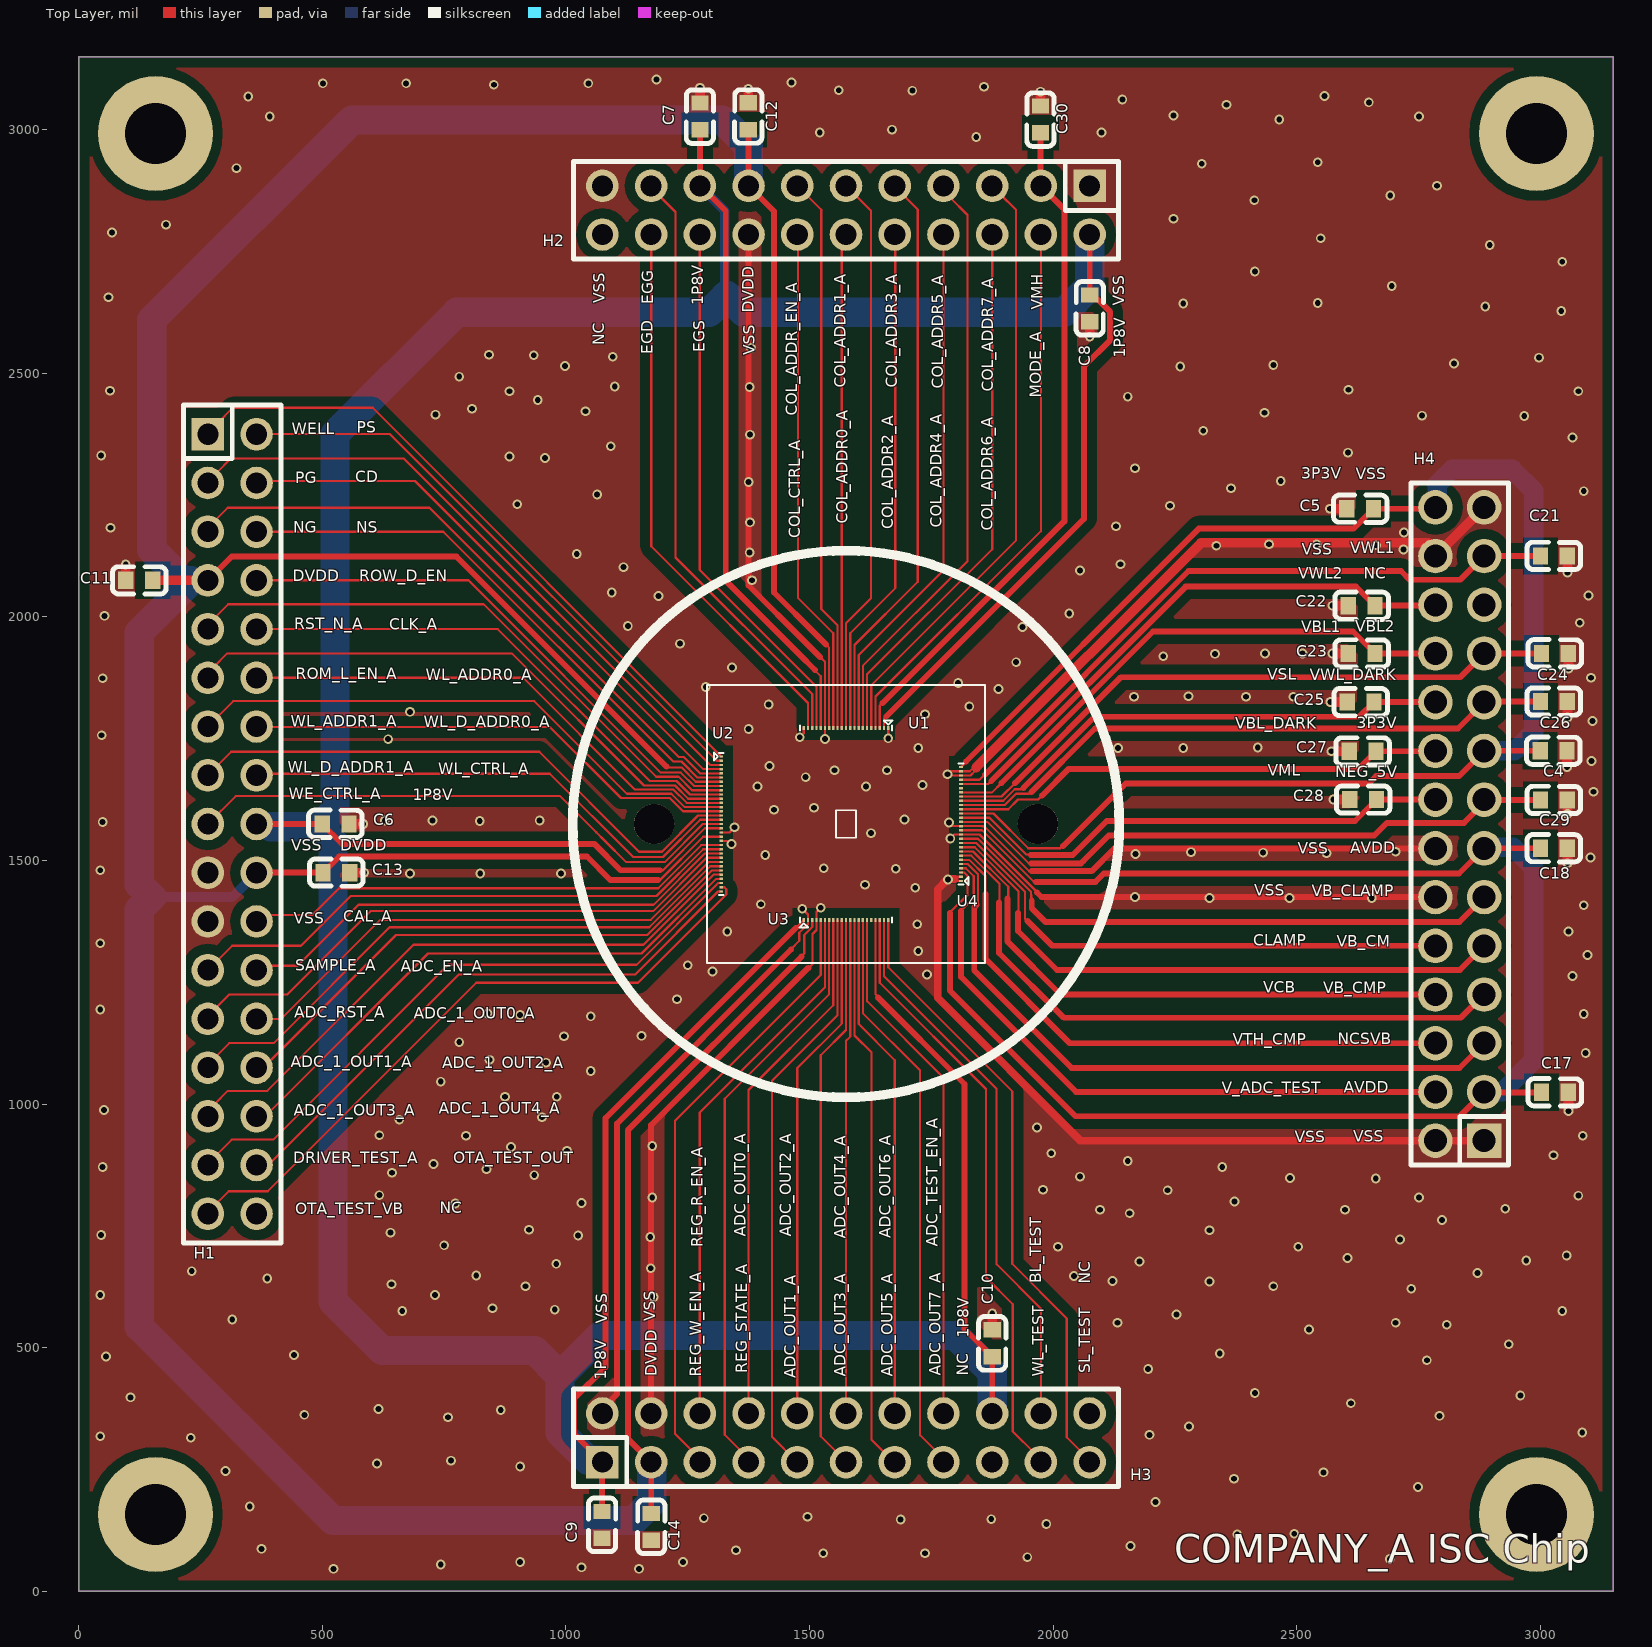
[diagram p0: Top Layer view]
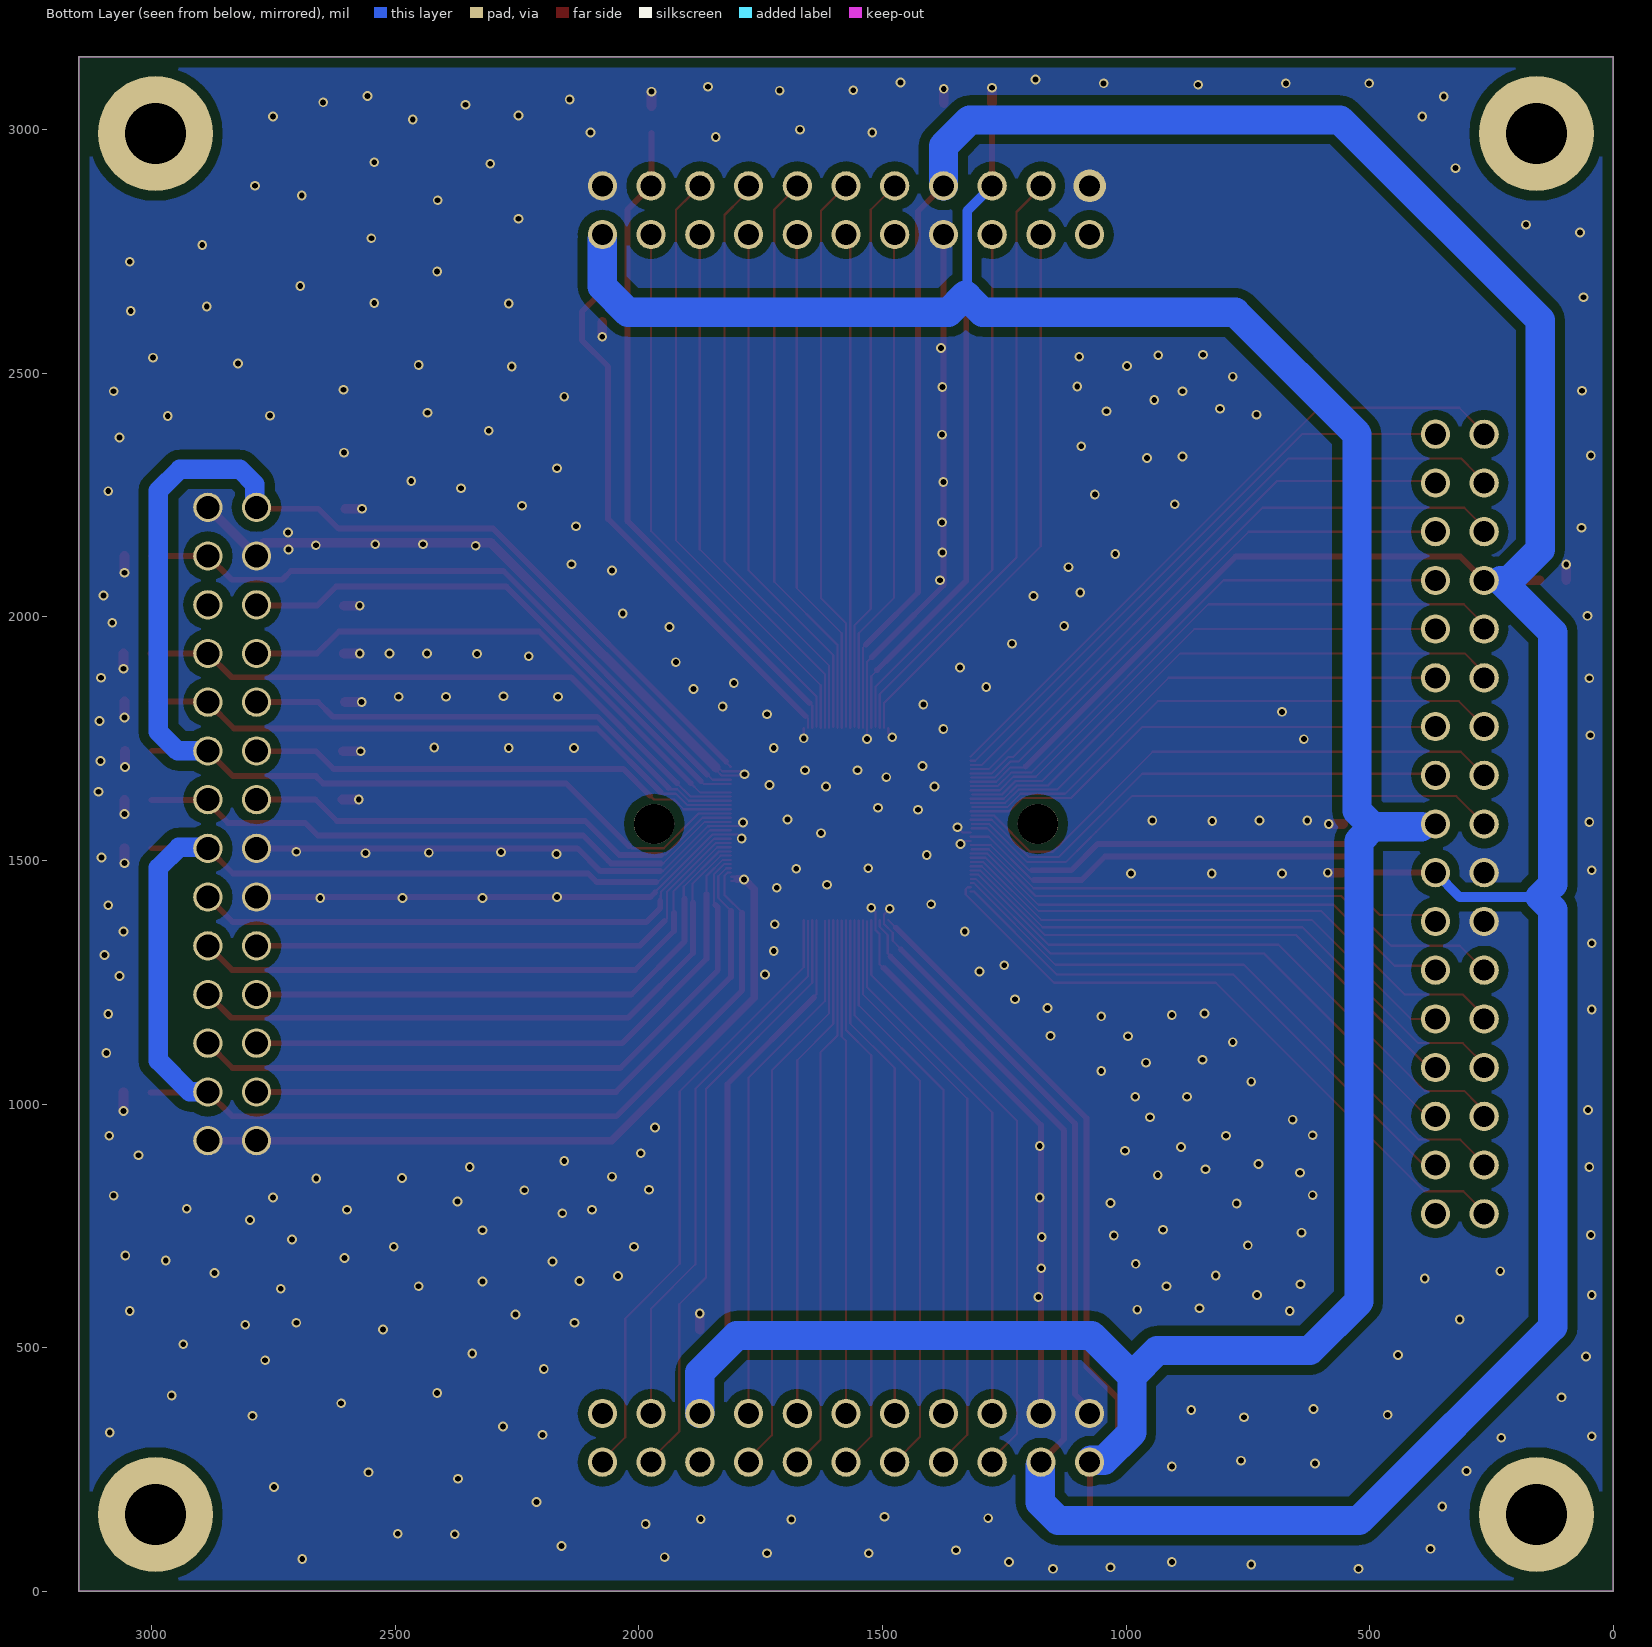
[diagram p1: Bottom Layer view, seen from below]
# Altium PCB MISC79019.PcbDoc
Units mil, origin at the board's own origin, x right, y up, seen from the top; angles counter-clockwise.
Board outline 3149.61 x 3149.61 mil, 2 copper layers (Top Layer, Bottom Layer); 31 components, 80 nets, 261 pads, 355 vias.

## Layer stack, top to bottom (the 12.6 mil dielectric is the usual default, probably not edited)
Top Layer: signal copper 1.4
Dielectric: dielectric 12.6, FR-4, Dk 4.8
Bottom Layer: signal copper 1.4

## Board outline
0,0 3149.61,0 3149.61,3149.61 0,3149.61

## Design rules (kind name [scope] priority, off if disabled: settings)
Clearance Clearance_2 [inpolygon] p1: gap=20
Clearance Clearance_1 [ispad vs ispad] p2: gap=3
Clearance [All] p3: gap=4
HoleSize [All] p1: absolutevalues=TRUE maxlimit=500 minlimit=1 maxpercent=80.000 minpercent=20.000
HoleToHoleClearance [All] p1: gap=0 allowstackedmicrovias=TRUE
MinimumSolderMaskSliver [All] p1: minsoldermaskwidth=0
PlaneClearance [All] p1: clearance=6
PlaneConnect [All] p1: planeconnectstyle=Direct reliefexpansion=20 reliefentries=4 reliefconductorwidth=10 reliefairgap=10
PolygonConnect [All] p1: connectstyle=Direct reliefconductorwidth=10 reliefentries=4 polygonreliefangle="90 Angle"
RoutingVias [All] p1: holewidth=12 width=20 viastyle="Through Hole" minholewidth=12 minwidth=20 maxholewidth=12 maxwidth=20
SilkToSilkClearance [All] p1: silktosilkclearance=0
SilkscreenOverComponentPads [All] p1: minsilkscreentomaskgap=0
SolderMaskExpansion [All] p1: expansion=4
Width [All] p1: maxlimit=80 minlimit=4 preferedwidth=4 minimp=50.000000 maximp=50.000000 favimp=50.000000
21 further rules are at their usual default settings.

## Components (designator, comment, footprint, x,y, rotation, side; value= is the part's Value field where it differs from the comment)
C4 "100nF/16V" 0603C 3027,1725 r0 top
C5 "100nF/16V" 0603C 2630,2222 r180 top
C6 "100nF/16V" 0603C 527,1575 r0 top
C7 "100nF/16V" 0603C 1275,3027 r90 top
C8 "100nF/16V" 0603C 2075,2633 r270 top
C9 "100nF/16V" 0603C 1074,136 r270 top
C10 "100nF/16V" 0603C 1875,509 r90 top
C11 "100nF/16V" 0603C 124,2075 r180 top
C12 "100nF/16V" 0603C 1374.3,3027.3 r90 top
C13 "100nF/16V" 0603C 529,1475 r0 top
C14 "100nF/16V" 0603C 1175,132 r270 top
C17 "100nF/16V" 0603C 3030,1024 r0 top
C18 "100nF/16V" 0603C 3028,1525 r0 top
C21 "100nF/16V" 0603C 3028,2125 r0 top
C22 "100nF/16V" 0603C 2633,2023 r180 top
C23 "100nF/16V" 0603C 2633,1925 r180 top
C24 "100nF/16V" 0603C 3030,1925 r0 top
C25 "100nF/16V" 0603C 2631,1825 r180 top
C26 "100nF/16V" 0603C 3028,1826 r0 top
C27 "100nF/16V" 0603C 2635,1724 r180 top
C28 "100nF/16V" 0603C 2636,1625 r180 top
C29 "100nF/16V" 0603C 3028,1624 r0 top
C30 "100nF/16V" 0603C 1974,3021 r90 top
H1 "#NAME?" HDR-TH_34P-P2.54-V-M-R2-C17-S2.54 314.96,1574.8 r270 top locked
H2 "#NAME?" HDR-TH_22P-P2.54-V-M-R2-C11-S2.54#1 1574.8,2834.65 r180 top locked
H3 "#NAME?" HDR-TH_22P-P2.54-V-M-R2-C11-S2.54#2 1574.8,314.96 r0 top locked
H4 "#NAME?" HDR-TH_28P-P2.54-V-M-R2-C14-S2.54 2834.65,1574.8 r90 top locked
U1 "X6511WVS-21H-C60D48R2" JSZ21 1574.8,1771.65 r270 top
U2 "X6511WVS-33H-C60D48R2" JSZ33 1318.9,1574.8 r0 top
U3 "X6511WVS-21H-C60D48R2" JSZ21 1574.8,1377.95 r90 top
U4 "X6511WVS-28H-C60D48R1" JSZ28 1811.02,1574.8 r180 top

## Footprints (in the part's own frame and the unit in brackets; to place one, negate y for a bottom-side part, rotate by r counter-clockwise, add the part's x,y. Pads: shape width x height; smd on the part's side, far side on the other; paste and mask are expansions set on the pad)
0603C [mm]
  rect 0.8x0.9 smd: 1(-0.7,0) 2(0.7,0)
  silkscreen extent -1.41,-0.71 1.39,0.72
HDR-TH_22P-P2.54-V-M-R2-C11-S2.54#1 [mm]
  rect 1.7x1.7 / inner round 1.524 / far side round 1.524 hole 1.1: 1(-12.7,-1.27)
  round 1.7 / inner round 1.524 / far side round 1.524 hole 1.1: 2(-12.7,1.27) 3(-10.16,-1.27) 4(-10.16,1.27) 5(-7.62,-1.27) 6(-7.62,1.27) 7(-5.08,-1.27) 8(-5.08,1.27) 9(-2.54,-1.27) 10(-2.54,1.27) 11(0,-1.27) 12(0,1.27) 13(2.54,-1.27) 14(2.54,1.27) 15(5.08,-1.27) 16(5.08,1.27) 17(7.62,-1.27) 18(7.62,1.27) 19(10.16,-1.27) 20(10.16,1.27) 22(12.7,1.27)
  round 1.7 hole 1.1: 21(12.7,-1.27)
  silkscreen extent -14.2,-2.54 14.2,2.54
HDR-TH_22P-P2.54-V-M-R2-C11-S2.54#2 [mm]
  rect 1.7x1.7 / inner round 1.524 / far side round 1.524 hole 1.1: 1(-12.7,-1.27)
  round 1.7 / inner round 1.524 / far side round 1.524 hole 1.1: 2(-12.7,1.27) 3(-10.16,-1.27) 4(-10.16,1.27) 5(-7.62,-1.27) 6(-7.62,1.27) 7(-5.08,-1.27) 8(-5.08,1.27) 9(-2.54,-1.27) 10(-2.54,1.27) 11(0,-1.27) 12(0,1.27) 13(2.54,-1.27) 14(2.54,1.27) 15(5.08,-1.27) 16(5.08,1.27) 17(7.62,-1.27) 18(7.62,1.27) 19(10.16,-1.27) 20(10.16,1.27) 21(12.7,-1.27) 22(12.7,1.27)
  silkscreen extent -14.2,-2.54 14.2,2.54
HDR-TH_28P-P2.54-V-M-R2-C14-S2.54 [mm]
  rect 1.8x1.8 / inner round 1.524 / far side round 1.524 hole 1.2: 1(-16.51,-1.27)
  round 1.8 / inner round 1.524 / far side round 1.524 hole 1.2: 2(-16.51,1.27) 3(-13.97,-1.27) 4(-13.97,1.27) 5(-11.43,-1.27) 6(-11.43,1.27) 7(-8.89,-1.27) 8(-8.89,1.27) 9(-6.35,-1.27) 10(-6.35,1.27) 11(-3.81,-1.27) 12(-3.81,1.27) 13(-1.27,-1.27) 14(-1.27,1.27) 15(1.27,-1.27) 16(1.27,1.27) 17(3.81,-1.27) 18(3.81,1.27) 19(6.35,-1.27) 20(6.35,1.27) 21(8.89,-1.27) 22(8.89,1.27) 23(11.43,-1.27) 24(11.43,1.27) 25(13.97,-1.27) 26(13.97,1.27) 27(16.51,-1.27) 28(16.51,1.27)
  silkscreen extent -17.78,-2.54 17.78,2.54
HDR-TH_34P-P2.54-V-M-R2-C17-S2.54 [mm]
  rect 1.7x1.7 / inner round 1.524 / far side round 1.524 hole 1.1: 1(-20.32,-1.27)
  round 1.7 / inner round 1.524 / far side round 1.524 hole 1.1: 2(-20.32,1.27) 3(-17.78,-1.27) 4(-17.78,1.27) 5(-15.24,-1.27) 6(-15.24,1.27) 7(-12.7,-1.27) 8(-12.7,1.27) 9(-10.16,-1.27) 10(-10.16,1.27) 11(-7.62,-1.27) 12(-7.62,1.27) 13(-5.08,-1.27) 14(-5.08,1.27) 15(-2.54,-1.27) 16(-2.54,1.27) 17(0,-1.27) 18(0,1.27) 19(2.54,-1.27) 20(2.54,1.27) 21(5.08,-1.27) 22(5.08,1.27) 23(7.62,-1.27) 24(7.62,1.27) 25(10.16,-1.27) 26(10.16,1.27) 27(12.7,-1.27) 28(12.7,1.27) 29(15.24,-1.27) 30(15.24,1.27) 31(17.78,-1.27) 32(17.78,1.27) 33(20.32,-1.27) 34(20.32,1.27)
  silkscreen extent -21.84,-2.54 21.84,2.54
JSZ21 [mm]
  rect 0.2x0.12 smd: 1(0,2.2) 2(0,1.98) 3(0,1.76) 4(0,1.54) 5(0,1.32) 6(0,1.1) 7(0,0.88) 8(0,0.66) 9(0,0.44) 10(0,0.22) 11(0,0) 12(0,-0.22) 13(0,-0.44) 14(0,-0.66) 15(0,-0.88) 16(0,-1.1) 17(0,-1.32) 18(0,-1.54) 19(0,-1.76) 20(0,-1.98) 21(0,-2.2)
  silkscreen extent -0.39,-2.39 0.13,2.42
JSZ28 [mm]
  rect 0.2x0.12 smd: 1(0,2.97) 2(0,2.75) 3(0,2.53) 4(0,2.31) 5(0,2.09) 6(0,1.87) 7(0,1.65) 8(0,1.43) 9(0,1.21) 10(0,0.99) 11(0,0.77) 12(0,0.55) 13(0,0.33) 14(0,0.11) 15(0,-0.11) 16(0,-0.33) 17(0,-0.55) 18(0,-0.77) 19(0,-0.99) 20(0,-1.21) 21(0,-1.43) 22(0,-1.65) 23(0,-1.87) 24(0,-2.09) 25(0,-2.31) 26(0,-2.53) 27(0,-2.75) 28(0,-2.97)
  silkscreen extent -0.39,-3.16 0.13,3.19
JSZ33 [mm]
  rect 0.2x0.12 smd: 1(0,3.52) 2(0,3.3) 3(0,3.08) 4(0,2.86) 5(0,2.64) 6(0,2.42) 7(0,2.2) 8(0,1.98) 9(0,1.76) 10(0,1.54) 11(0,1.32) 12(0,1.1) 13(0,0.88) 14(0,0.66) 15(0,0.44) 16(0,0.22) 17(0,0) 18(0,-0.22) 19(0,-0.44) 20(0,-0.66) 21(0,-0.88) 22(0,-1.1) 23(0,-1.32) 24(0,-1.54) 25(0,-1.76) 26(0,-1.98) 27(0,-2.2) 28(0,-2.42) 29(0,-2.64) 30(0,-2.86) 31(0,-3.08) 32(0,-3.3) 33(0,-3.52)
  silkscreen extent -0.39,-3.71 0.13,3.74

## Part data
C4 C5 C6 C7 C8 C9 C10 C11 C12 C13 C14 C17 C18 C21 C22 C23 C24 C25 C26 C27 C28 C29 C30: library part CAP, "component CAP componentdescr capacitor model"
H1: library part PZ254-2-17-Z-8.5
H2 H3: library part PZ254-2-11-Z-8.5
H4: library part PZ254-2-14-Z-8.5

## Free pads (board coordinates)
  round 82.68 hole 82.68 unplated: 0(1181.1,1574.8) 0(1968.5,1574.8)
  round 236.22 hole 125.98: 2(157.48,157.48) 2(157.48,2992.13) 2(2992.13,157.48) 2(2992.13,2992.13)

## Via types
v1: diameter 20, hole 12, Top Layer to Bottom Layer, tented both sides, 355 vias

## Nets (pads, with @x,y where several pads share a name; then routed paths per layer and width w, separated by ;. In a path a pad name is that pad's centre, name@x,y a point inside that pad or via, vN(x,y) a via of type N, cw(c..) or ccw(c..) an arc to the next point about the centre after c; other vN are vias at no path point)
1P8V: C6.1 C7.1 C8.1 C9.1 C10.1 H1.18 H2.2 H2.17 H3.1 H3.18 U1.2 U1.17 U2.18 U3.1 U3.18 | length 11858.5
  Top Layer w4.5: 1193,1480 1199,1480 1285.09,1566.09 U2.18@1317,1566.09 ; 1472,1362 1472.24,1362 U3.1 ; 1496,1905 1522.83,1878.17 U1.17 ; U3.18 1635.43,1225.57 1639,1222 ; U1.2 1652.76,1791.76 1657,1796
  Top Layer w12: H1.18 C6.1@494.8,1574.8 ; C6.1 540.44,1534 1058,1534 1112,1480 1193,1480 ; C9.1 H3.1@1074,250 ; H3.1 1017,322.76 1017,396 1081,460 1081,971 1472,1362 ; C7.1 1275,2886 1328,2833 1328,2074 1478,1924 ; 1487,1915 1478,1924 ; 1511,1891 1478,1924 ; 1640,1219 1818,1041 1818,538.44 C10.1 H3.18@1875,366 ; 1658,1796 2063,2201 2063,2514 2117,2568 2117,2626 2082.44,2660.56 C8.1 H2.2@2075,2760
  Bottom Layer w20: H2.17 1326,2833.45 1326,2657
  Bottom Layer w60: H1.18@394,1569 493,1569 ; H3.1@1072,269 1045,269 988,326 988,442 ; H3.18 1874.8,449.2 1799,525 1071,525 988,442 ; H2.2@2075,2775 2075,2678 2022,2625 1365,2625 1329.5,2660.5 1326,2657 1294,2625 776,2625 526,2375 526,1602 493,1569 ; 493,1569 522,1540 522,595 623,494 936,494 988,442
3P3V: C4.1 C5.1 H4.17 H4.28 U4.17 U4.28 | length 3336.5
  Top Layer w4.5: U4.17 1877.54,1596.46 1949,1525 2015,1525 2020,1530 ; U4.28@1812.73,1691.73 U4.28 1820,1700.71 1820,1702
  Top Layer w12: 1821,1703 2299,2181 2616.56,2181 C5.1 H4.28@2764,2222 ; 2020.5,1529.5 2149,1658 2648,1658 2663,1673 2832.84,1673 H4.17 ; H4.17@2895,1725 C4.1
  Bottom Layer w40: H4.28@2788,2241 2788,2272 2819,2303 2942,2303 2986,2259 2986,1764 2946.8,1724.8 H4.17
ADC_1_OUT0_A: H1.26 U2.26 | length 1087.3
  Top Layer w4.5: H1.26 415.8,1174.8 619,1378 1173.94,1378 1292.79,1496.85 U2.26
ADC_1_OUT1_A: H1.27 U2.27 | length 1195.7
  Top Layer w4.5: H1.27@284,1100 309,1125 400,1125 638,1363 1170.96,1363 1296.15,1488.19 U2.27
ADC_1_OUT2_A: H1.28 U2.28 | length 1108.9
  Top Layer w4.5: H1.28@378,1074 651,1347 1166.98,1347 1299.51,1479.53 U2.28
ADC_1_OUT3_A: H1.29 U2.29 | length 1234.9
  Top Layer w4.5: H1.29@279,1000 306,1027 387,1027 687,1327 1159,1327 1302.87,1470.87 U2.29
ADC_1_OUT4_A: H1.30 U2.30 | length 1141.9
  Top Layer w4.5: H1.30@380,972 717,1309 1155,1309 1308.2,1462.2 U2.30
ADC_EN_A: H1.24 U2.24 | length 1027.2
  Top Layer w4.5: H1.24@387,1284 449,1284 574,1409 1179.98,1409 1285.15,1514.17 U2.24
ADC_OUT0_A: H3.8 U3.8 | length 1084.1
  Top Layer w4.5: H3.8 1374.8,1028.8 1548.77,1202.77 U3.8@1548.77,1377
ADC_OUT1_A: H3.9 U3.9 | length 1188.8
  Top Layer w4.5: H3.9@1474,266 1423,317 1423,1048 1557.48,1182.48 U3.9
ADC_OUT2_A: H3.10 U3.10 | length 1049.9
  Top Layer w4.5: H3.10 1474.8,1073.8 1566.09,1165.09 U3.10@1566.09,1377
ADC_OUT3_A: H3.11 U3.11 | length 1146.5
  Top Layer w4.5: H3.11@1569,272 1523,318 1523,1100 1574.8,1151.8 U3.11
ADC_OUT4_A: H3.12 U3.12 | length 1015.6
  Top Layer w4.5: H3.12 1574.8,1129.8 1583.42,1138.42 U3.12@1583.42,1377
ADC_OUT5_A: H3.13 U3.13 | length 1128.1
  Top Layer w4.5: U3.13 1592.13,1140.87 1627,1106 1627,311 H3.13@1660,278
ADC_OUT6_A: H3.14 U3.14 | length 1043.7
  Top Layer w4.5: U3.14 1600.84,1164.16 1674.8,1090.2 H3.14
ADC_OUT7_A: H3.15 U3.15 | length 1160.4
  Top Layer w4.5: U3.15 1609.45,1186.55 1727,1069 1727,320 H3.15@1765,282
ADC_RST_A: H1.25 U2.25 | length 1172.8
  Top Layer w4.5: H1.25@276,1192 309,1225 428,1225 599,1396 1179,1396 1288.51,1505.51 U2.25
ADC_TEST_EN_A: H3.16 U3.16 | length 1076.9
  Top Layer w4.5: U3.16@1618.16,1377 1618.16,1210.84 1774.8,1054.2 H3.16
AVDD: C17.1 C18.1 H4.3 H4.13 U4.3 U4.13 | length 3477.4
  Top Layer w4.5: 1786,1391 1824,1429 1824,1468.7 1817.5,1475.2 U4.3 ; U4.13 1854.19,1561.81 1960,1456 1965,1456
  Top Layer w12: 1788,1392 1788,1233 2046,975 2834.84,975 H4.3 ; 1965,1456 2087,1456 2104,1473 2155,1473 ; 2146,1473 2155,1473 ; H4.13 2832.84,1473 2155,1473 ; H4.13@2901,1525 C18.1 ; H4.3@2904,1024 C17.1
  Bottom Layer w40: H4.3 2921.8,1024.8 2986,1089 2986,1485 2944,1527 H4.13@2895,1527
BL_TEST: H3.20 U3.20 | length 1145.4
  Top Layer w4.5: U3.20@1652.81,1377 1652.81,1262.19 1884,1031 1884,671 1974.8,580.2 H3.20
CAL_A: H1.22 U2.22 | length 991.3
  Top Layer w4.5: H1.22@387,1388 479,1388 534,1443 1189.32,1443 1277.82,1531.5 U2.22
CD: H1.4 U2.4 | length 1179.9
  Top Layer w4.5: H1.4@384,2279 690,2279 1281.6,1687.4 U2.4
CLK_A: H1.10 U2.10 | length 1091.6
  Top Layer w4.5: H1.10 860.2,1974.8 1172,1663 1227,1663 1254.52,1635.48 U2.10@1316,1635.48
COL_ADDR0_A: H2.12 U1.12 | length 1000.7
  Top Layer w4.5: U1.12 1566.14,2771.14 H2.12@1567,2772
COL_ADDR1_A: H2.11 U1.11 | length 1153
  Top Layer w4.5: H2.11 1626,2833.45 1626,2038 1574.85,1986.85 U1.11@1574.85,1774
COL_ADDR2_A: H2.10 U1.10 | length 1039.7
  Top Layer w4.5: U1.10 1583.46,1966.46 1676,2059 H2.10@1676,2773
COL_ADDR3_A: H2.9 U1.9 | length 1163.4
  Top Layer w4.5: U1.9 1592.13,1942.13 1722,2072 1722,2836 H2.9@1690,2868
COL_ADDR4_A: H2.8 U1.8 | length 1082.7
  Top Layer w4.5: U1.8@1600.84,1774 1600.84,1921.84 1774.8,2095.8 H2.8
COL_ADDR5_A: H2.7 U1.7 | length 1193.1
  Top Layer w4.5: U1.7 1609.45,1899.45 1824,2114 1824,2825 H2.7@1788,2861
COL_ADDR6_A: H2.6 U1.6 | length 1119
  Top Layer w4.5: U1.6@1618.06,1772 1618.06,1882.06 1874.8,2138.8 H2.6
COL_ADDR7_A: H2.5 U1.5 | length 1233.1
  Top Layer w4.5: U1.5 1626.77,1859.77 1924,2157 1924,2835 H2.5@1891,2868
COL_ADDR_EN_A: H2.13 U1.13 | length 1144.9
  Top Layer w4.5: H2.13 1524,2835.45 1524,2016 1557.53,1982.47 U1.13@1557.53,1774
COL_CTRL_A: H2.14 U1.14 | length 1034.5
  Top Layer w4.5: H2.14@1476,2776 1476,2039 1548.82,1966.18 U1.14
DRIVER_TEST_A: H1.31 U2.31 | length 1278.2
  Top Layer w4.5: H1.31@275,888 314,927 399,927 758,1286 1145,1286 1308.71,1449.71 1308.71,1449.83 1312.42,1453.54 U2.31
DVDD: C11.1 C12.1 C13.1 C14.1 H1.7 H1.20 H2.15 H3.3 U1.15 U2.7 U2.20 U3.3 | length 10270.4
  Top Layer w4.5: 1189,1461 1194,1461 1281.82,1548.82 U2.20 ; 1208,1694 1211,1691 1236.98,1691 1266.56,1661.42 U2.7 ; 1483,1303 1489,1309 1489,1347 1505.51,1363.51 U3.3 ; 1528,1945 1534,1939 ; 1536,1941 1540.16,1936.84 1540.16,1932.84 1540.16,1930 U1.15
  Top Layer w12: H1.7 314.16,2124 775,2124 1206.5,1692.5 ; H1.20@364,1475 C13.1 534.44,1508 1043,1508 1091,1460 1189,1460 ; H3.3 1127,312.76 1127,946 1483.5,1302.5 ; C14.1 H3.3@1175,244 ; C12.1@1374.8,2993.2 H2.15 1427,2832.45 1427,2050 1512.5,1964.5 ; 1517,1960 1512.5,1964.5 ; 1534,1943 1512.5,1964.5
  Top Layer w20: C11.1 H1.7@254,2075
  Bottom Layer w20: 148,1425 150,1425 315.16,1425 H1.20
  Bottom Layer w60: 213,2075 150,2138 150,2609 561,3020 1321,3020 1374.8,2966.2 H2.15 ; 230.8,2074.8 124,1968 124,1451 150,1425 124,1399 124,543 522,145 1139,145 1176,182 H3.3@1176,258
EGD: H2.20 U1.20 | length 1132.7
  Top Layer w4.5: H2.20@1175,2771 1175,2145 1496.85,1823.15 U1.20
EGG: H2.19 U1.19 | length 1227.9
  Top Layer w4.5: H2.19@1188,2868 1225,2831 1225,2122 1505.51,1841.49 U1.19
EGS: H2.18 U1.18 | length 1109.8
  Top Layer w4.5: H2.18 1274.8,2096.2 1514.22,1856.78 U1.18@1514.22,1774
MODE_A: H2.4 U1.4 | length 1151.2
  Top Layer w4.5: U1.4@1635.38,1774 1635.38,1836.38 1974.8,2175.8 H2.4
NCSVB: H4.5 U4.5 | length 1394.7
  Top Layer w4.5: U4.5 1824.46,1492.52 1846,1470.98 1846,1412 1843,1409
  Top Layer w12: 1843,1409 1838,1404 1838,1274 2038,1074 2833.84,1074 H4.5
NEG_5V: C29.1 H4.15 U4.15 | length 1281.5
  Top Layer w4.5: U4.15 1864.87,1579.13 1950,1494 1957,1494 ; 2062,1499 2063,1499
  Top Layer w12: 1955,1494 1957,1494 2057,1494 2062,1499 2114,1551 2659,1551 2685,1577 2843,1577 2890,1624 C29.1
NG: H1.5 U2.5 | length 1282.5
  Top Layer w4.5: H1.5@275,2193 306,2224 720,2224 1231.5,1712.5 1241.5,1712.5 1275,1679 ; 1275,1678.74 U2.5
NS: H1.6 U2.6 | length 1162.1
  Top Layer w4.5: H1.6 748.2,2174.8 1220,1703 1237,1703 1269.97,1670.03 U2.6@1318,1670.03
OTA_TEST_OUT: H1.32 U2.33 | length 1199.7
  Top Layer w4.5: H1.32@378,878 392,878 426.5,912.5 ; 407,893 426.5,912.5 ; U2.33 1312.22,1436.22 1142,1266 780,1266 426.5,912.5
OTA_TEST_VB: H1.33 U2.32 | length 1340
  Top Layer w4.5: H1.33@277,790 308,821 388,821 816,1249 1148,1249 1329.08,1430.08 1329.08,1441.17 1325.37,1444.88 U2.32
PG: H1.3 U2.3 | length 1309.8
  Top Layer w4.5: H1.3@282,2295 312,2325 667,2325 1295.94,1696.06 U2.3
PS: H1.2 U2.2 | length 1214.5
  Top Layer w4.5: H1.2@382,2375 639,2375 1309.28,1704.72 U2.2
REG_R_EN_A: H3.6 U3.6 | length 1117.4
  Top Layer w4.5: H3.6 1274.8,982.8 1531.55,1239.55 U3.6@1531.55,1376
REG_STATE_A: H3.7 U3.7 | length 1203.6
  Top Layer w4.5: H3.7@1367,280 1326,321 1326,1011 1540.16,1225.16 U3.7
REG_W_EN_A: H3.5 U3.5 | length 1236.7
  Top Layer w4.5: H3.5@1265,282 1224,323 1224,966 1522.83,1264.83 U3.5
ROW_D_EN_A: H1.8 U2.8 | length 1115.8
  Top Layer w4.5: H1.8@378,2075 800,2075 1194.75,1680.25 1235.71,1680.25 1263.2,1652.76 U2.8
ROW_L_EN_A: H1.11 U2.11 | length 1178.4
  Top Layer w4.5: H1.11@276,1896 305,1925 889,1925 1160,1654 1223.98,1654 1251.21,1626.77 U2.11
RST_N_A: H1.9 U2.9 | length 1226.7
  Top Layer w4.5: H1.9@267,1986 307,2026 831,2026 1185.25,1671.75 1231.25,1671.75 1258.91,1644.09 U2.9
SAMPLE_A: H1.23 U2.23 | length 1154.8
  Top Layer w4.5: H1.23 315.16,1325 456,1325 558,1427 1185.96,1427 1281.84,1522.88 U2.23@1317,1522.88
SL_TEST: H3.21 U3.21 | length 1284.5
  Top Layer w4.5: U3.21 1661.42,1280.58 1916,1026 1916,672 2028,560 2028,316 H3.21@2078,266
V_ADC_TEST: H4.4 U4.4 | length 1321.6
  Top Layer w4.5: 1811,1396 1811,1397 1837,1423 1837,1467.72 1820.86,1483.86 U4.4
  Top Layer w12: 1811,1396 1811,1261 2047.2,1024.8 H4.4
VB_CLAMP: H4.11 U4.11 | length 1183.7
  Top Layer w4.5: U4.11 1845.59,1544.49 1954.75,1435.33 1954.75,1428.68 1955,1428.43 1955,1418
  Top Layer w12: 1956,1418 1956,1402 1984,1374 2833.84,1374 H4.11
VB_CM: H4.9 U4.9 | length 1254.8
  Top Layer w4.5: U4.9 1838.88,1527.17 1929,1437.04 1929,1396
  Top Layer w12: 1928,1392 1928,1355 2008,1275 2187,1275 ; 2176,1275 2187,1275 ; H4.9 2834.84,1275 2187,1275
VB_CMP: H4.7 U4.7 | length 1328.5
  Top Layer w4.5: U4.7 1832.16,1509.84 1890,1452 1890,1414
  Top Layer w12: 1889,1414 1889,1310 2022,1177 2209,1177 ; 2196,1177 2209,1177 ; H4.7 2836.84,1177 2209,1177
VBL1: C23.1 H4.22 U4.22 | length 1117.4
  Top Layer w4.5: U4.22 1874.76,1639.76 1894,1659
  Top Layer w12: 1894,1659 2205,1970 2615.56,1970 C23.1 H4.22@2773,1925
VBL2: C24.1 H4.21 U4.21 | length 1296.7
  Top Layer w4.5: U4.21 1894.1,1631.1 1922,1659
  Top Layer w12: 1922,1659 2139,1876 2835.84,1876 H4.21 ; H4.21@2901,1925 C24.1
VBL_DARK: C27.1 H4.18 U4.18 | length 1010.8
  Top Layer w4.5: U4.18 1908.12,1605.12 1928,1625 1969,1625 1976,1632
  Top Layer w12: 1977,1633 2032,1688 2626.56,1688 C27.1 H4.18@2774,1724
VCB: H4.8 U4.8 | length 1162.9
  Top Layer w4.5: U4.8 1835.52,1518.5 1908,1446.02 1908,1422
  Top Layer w12: 1906,1422 1906,1334 2015.2,1224.8 H4.8
VCLAMP: H4.10 U4.10 | length 1124.5
  Top Layer w4.5: U4.10 U4.10@1813,1535.83 ; U4.10@1813,1535.78 1842.28,1535.78 1942,1436.06 1942,1381 1947,1376
  Top Layer w12: 1947,1376 1998.2,1324.8 2203,1324.8 ; 2171.8,1324.8 2203,1324.8 ; H4.10 2203,1324.8
VMH: C30.1 H2.3 U1.3 | length 1395.6
  Top Layer w4.5: U1.3 1644.09,1818.09 1649.5,1823.5
  Top Layer w12: 1650,1823 2023,2196 2023,2836.45 H2.3 ; H2.3@1974,2888 C30.1
VML: C28.1 H4.16 U4.16 | length 1036.5
  Top Layer w4.5: U4.16 1869.2,1587.8 1945,1512 1954,1512
  Top Layer w12: 1954,1511.25 2040.25,1511.25 2110,1581 2619.56,1581 C28.1 H4.16@2769,1625
VSL: C25.1 H4.20 U4.20 | length 1049.9
  Top Layer w4.5: U4.20 1897.46,1622.44 1921.02,1646 1936,1646 1939,1649
  Top Layer w12: 1939,1649 2085,1795 2628.56,1795 C25.1 H4.20@2777,1825
VSS: C4.2 C5.2 C6.2 C7.2 C8.2 C9.2 C10.2 C11.2 C12.2 C13.2 C14.2 C17.2 C18.2 C21.2 C22.2 C23.2 C24.2 C25.2 C26.2 C27.2 C28.2 C29.2 C30.2 H1.19 H1.21 H2.1 H2.16 H2.21 H3.2 H3.4 H4.1 H4.2 H4.12 H4.14 H4.26 H4.27 U1.1 U1.16 U1.21 U2.19 U2.21 U3.2 U3.4 U4.1 U4.2 U4.12 U4.14 U4.26 U4.27 | length 9321.6
  Top Layer w4.5: U2.21 1333.84,1540.16 v1(1340,1534) ; U2.19 1335.48,1557.48 v1(1346,1568) ; 1463,1319 1479,1335 1479,1351.68 1496.85,1369.53 U3.2 1496.85,1389.15 v1(1485,1401) ; v1(1480,1753) 1488.19,1761.19 U1.21 ; 1498,1279 1506,1287 1506,1349 1514.17,1357.17 U3.4 1514.17,1394.17 v1(1523,1403) ; 1521,1919 1531.5,1908.5 U1.16 v1(1531.5,1749.5) ; v1(1661.42,1750.58) U1.1 ; v1(1783,1677) 1789.07,1683.07 U4.27 1829.07,1683.07 1834,1688 ; v1(1786,1578) 1793.53,1570.47 U4.14 1853.53,1570.47 1853.69,1570.31 1858.69,1570.31 1951,1478 1956,1478 ; v1@1786,1674.41 U4.26 1830.41,1674.41 1840,1684 ; v1(1789,1545) 1797.15,1553.15 U4.12 1848.95,1553.15 1966,1436.1 1966,1435 ; 1799,1464 1801.54,1466.54 U4.2 ; 1801,1459 1802.13,1457.87 U4.1
  Top Layer w12: H3.2 1074.8,374.8 1105,405 1105,960 1462,1317 ; H3.4 1174.8,956.8 1497.5,1279.5 ; H2.16 1374.8,2064.2 1491,1948 ; 1496,1943 1491,1948 ; 1522,1917 1491,1948 ; 1956,1478 2079,1478 2125.8,1524.8 H4.14 ; 1967,1434 1976.2,1424.8 H4.12
  Top Layer w16: v1(1784,1461) v1@1784,1462 ; 1798,1462 v1@1784,1462 ; H4.1 H4.2 2056.2,924.8 1763,1218 1763,1441 v1@1784,1462
  Top Layer w20: C11.2 v1(96.44,2107.56) ; C6.2 v1(584,1575) ; C13.2 v1(586,1475) ; C7.2 v1(1275,3086) ; C12.2 v1(1374.3,3083.7) ; 1842,1691 2303,2152 2769.84,2152 2790.84,2131 H4.27 ; C10.2 v1(1875,570) ; C30.2 v1(1974,3078) ; v1(2075,2575) C8.2 ; v1(2568,2222) C5.2 ; v1(2569,1825) C25.2 ; v1(2571,1724) C27.2 ; v1(2573,1925) C23.2 ; v1(2573,2023) C22.2 ; v1(2575,1625) C28.2 ; v1(3054.56,1691.56) C4.2 ; v1(3055.56,1494.44) C18.2 ; v1(3055.56,1595.56) C29.2 ; v1(3055.56,1793.44) C26.2 ; v1(3055.56,2090.56) C21.2 ; v1(3057.56,985.56) C17.2 ; v1(3057.56,1893.56) C24.2
  other v1: 523,46 1150,46 1032,49 743,55 906,60 1240,60 2691,66 1947,70 1528,78 1737,78 1349,84 375,87 2159,93 2378,117 2495,118 1986,138 1687,147 1873,148 1283,150 1496,153 351,174 2210,183 2749,214 2371,231 2555,244 301,247 906,256 612,262 764,268 230,315 44,318 2198,321 3086,326 2279,338 758,357 2793,360 463,362 866,372 615,374 2611,386 106,398 2959,402 2414,407 2195,456 2767,474 56,482 442,485 2342,488 2935,507 2525,537 2808,547 2132,551 2703,551 315,558 2253,568 664,575 3045,575 977,578 849,581 1180,604 44,608 731,608 2735,621 917,626 2452,626 642,630 2321,636 2122,637 387,642 2043,647 816,648 2871,653 232,657 1174,663 980,672 2177,677 2971,679 2604,684 3054,689 2010,707 2503,707 750,710 2712,722 1173,727 1025,730 46,731 640,736 2321,741 924,742 2798,762 2157,776 2096,783 2599,783 2928,785 773,796 1032,797 2372,800 1177,808 2751,808 3078,812 617,813 2235,823 1979,824 2662,847 2486,848 2055,851 935,854 643,859 837,866 49,871 2347,871 728,877 2153,883 3027,895 1996,899 1002,904 887,912 1177,914 795,935 3087,935 617,936 1967,952 658,968 951,973 52,988 875,1015 981,1015 743,1046 1051,1068 959,1085 843,1091 3093,1105 781,1127 996,1139 1155,1140 1051,1180 906,1183 3089,1185 839,1186 44,1194 1161,1197 1228,1215 3066,1263 1741,1266 1301,1272 1250,1285 3097,1306 1723,1314 44,1330 1331,1354 3058,1354 1721,1369 3089,1408 1400,1410 2321,1423 2485,1423 2654,1423 2168,1425 1717,1444 1614,1450 680,1473 824,1473 990,1473 44,1480 1677,1483 1529,1484 3103,1506 1409,1511 2169,1513 2561,1515 2431,1516 2283,1517 2703,1518 1626,1556 49,1579 823,1581 628,1582 726,1582 946,1582 1695,1584 1427,1604 1509,1608 3109,1641 1393,1652 1616,1652 1732,1655 1492,1671 1551,1685 1659,1685 1418,1694 3105,1704 1723,1731 2133,1731 2267,1731 2420,1732 635,1749 47,1757 1375,1770 3107,1786 1737,1800 680,1805 1828,1816 1416,1820 2166,1836 2396,1836 2493,1836 2278,1837 1888,1852 1287,1856 1805,1864 49,1874 3104,1875 1341,1896 1924,1907 2226,1919 2332,1924 2435,1925 2512,1925 1234,1945 1937,1979 1127,1981 3081,1988 53,2002 2033,2007 1190,2043 3099,2044 1094,2050 1382,2075 2055,2095 1118,2102 2138,2108 1022,2129 1377,2132 2719,2138 2335,2146 2663,2147 2443,2149 2541,2149 2720,2173 65,2183 2129,2186 1378,2194 2240,2228 900,2231 1064,2251 3089,2258 2365,2264 1375,2277 2467,2279 2168,2305 957,2326 884,2329 46,2331 2605,2337 1092,2350 3066,2368 1378,2374 2308,2382 2967,2412 2757,2413 732,2415 2434,2419 1040,2422 807,2427 942,2445 2153,2452 884,2463 3078,2463 64,2464 2606,2466 1377,2472 1100,2473 781,2493 2261,2514 998,2515 2452,2517 2823,2520 2997,2532 1096,2534 934,2537 842,2538 1380,2552 3043,2628 2887,2637 2267,2643 2543,2644 61,2656 2695,2679 2414,2709 3045,2729 2896,2763 2549,2777 68,2789 179,2805 2247,2817 2413,2855 2692,2865 2788,2885 324,2921 2305,2930 2543,2933 1842,2985 1521,2994 2099,2994 1669,3000 2464,3021 392,3027 2751,3027 2247,3029 2356,3051 2648,3056 2142,3062 348,3068 2557,3069 1711,3080 1560,3081 1858,3088 852,3092 501,3095 672,3095 1046,3095 1463,3097 1186,3103
VTH_CMP: H4.6 U4.6 | length 1356.1
  Top Layer w4.5: U4.6 1827.82,1501.18 1861,1468 1861,1431 1861,1304
  Top Layer w12: 1861,1431 1861,1298 2034.2,1124.8 H4.6
VWL1: C21.1 H4.25 U4.25 | length 1384.7
  Top Layer w4.5: U4.25 1848.75,1665.75 1858,1675
  Top Layer w12: 1860,1676 2278,2094 2714,2094 2732,2076 2835.84,2076 H4.25 ; H4.25@2892,2125 C21.1
VWL2: C22.1 H4.24 U4.24 | length 1137.9
  Top Layer w4.5: U4.24 1867.09,1657.09 1873,1663
  Top Layer w12: 1873,1663 2272,2062 2621.56,2062 C22.1 H4.24@2765,2023
VWL_DARK: C26.1 H4.19 U4.19 | length 1251.9
  Top Layer w4.5: U4.19 1900.82,1613.78 1923.79,1636.75 1949.75,1636.75 1954,1641
  Top Layer w12: 1955,1640 2086,1771 2830.84,1771 H4.19 ; H4.19@2909,1826 C26.1
WE_CTRL_A: H1.17 U2.17 | length 1164.4
  Top Layer w4.5: H1.17 322.16,1632 988,1632 1062,1558 1079,1541 1123.5,1496.5 1202.5,1496.5 1280.96,1574.96 1312.26,1574.96 1312.37,1574.85 U2.17@1317,1574.85
WELL: H1.1 U2.1 | length 1343.2
  Top Layer w4.5: H1.1@285,2398 316,2429 603.28,2429 U2.1
WL_ADDR0_A: H1.12 U2.12 | length 1060.3
  Top Layer w4.5: H1.12 912.2,1874.8 1141.5,1645.5 1220.46,1645.5 1247.85,1618.11 U2.12
WL_ADDR1_A: H1.13 U2.13 | length 1162.8
  Top Layer w4.5: H1.13 317.16,1827 935,1827 1125,1637 1216,1637 1243.6,1609.4 U2.13@1316,1609.4
WL_CTRL_A: H1.16 U2.16 | length 1042.4
  Top Layer w4.5: H1.16@379,1678 967,1678 1138,1507 1199,1507 1275.46,1583.46 U2.16
WL_D_ADDR0_A: H1.14 U2.14 | length 998.6
  Top Layer w4.5: H1.14@392,1774 967,1774 1113,1628 1212.98,1628 1240.19,1600.79 U2.14
WL_D_ADDR1_A: H1.15 U2.15 | length 1187.6
  Top Layer w4.5: H1.15 313.16,1723 945,1723 1150,1518 1197,1518 1271.08,1592.08 U2.15@1317,1592.08
WL_TEST: H3.19 U3.19 | length 1226.6
  Top Layer w4.5: U3.19 1644.09,1248.91 1862,1031 1862,644 1917,589 1917,328 H3.19@1962,283
pads on no net: H1.34 H2.22 H3.17 H3.22 H4.23 U3.17 U4.23

## Polygon pours and split planes (outlines as drawn)
VSS on Top Layer "Bottom Layer-No Net" (solid, remove dead copper, pour order 1000): -229,2993 -253,2969 -253,-155 -133,-155 107,-395 179,-323 3243,-323 3244,-323 3484,-83 3544,-23 3544,3101 3544,3340 3435,3449 3338,3546 3003,3546 -24,3546 -193,3377 -217,3353 -217,2999
VSS on Bottom Layer "Bottom Layer-No Net" (solid, remove dead copper, pour order 1001): -217,2801 -217,-59 -37,-239 59,-335 251,-335 3207,-335 3363,-179 3411,-131 3411,-35 3411,3113 3255,3269 3171,3353 3027,3353 -28,3353 -187,3194 -217,3164 -217,2801

## Keep-outs
Keep-Out Layer:
  the board outline again, w3.94

## Silkscreen, mask and mechanical layers (free items; w line width, h text height)
Top Overlay:
  circle w19.68: c1574.8,1574.8 r561.02
  lines w3.94: 1289.37,1289.37 1289.37,1860.24 1860.24,1860.24 1860.24,1289.37 1289.37,1289.37 ; 1553.94,1546.65 1553.94,1602.95 1595.67,1602.95 1595.67,1546.65 1553.94,1546.65
  text "VSS" at 1088,2644 h40 r90
  text "EGG" at 1187,2642 h40 r90
  text "1P8V" at 1290,2640 h40 r90
  text "VSS" at 2154,2639 h40 r90
  text "VMH" at 1987,2630 h40 r90
  text "DVDD" at 1394,2624 h40 r90
  text "NC" at 1087,2557 h40 r90
  text "EGS" at 1293,2543 h40 r90
  text "EGD" at 1186,2539 h40 r90
  text "VSS" at 1396,2537 h40 r90
  text "1P8V" at 2156,2532 h40 r90
  text "COL_ADDR1_A" at 1583,2470 h40 r90
  text "COL_ADDR3_A" at 1688,2470 h40 r90
  text "COL_ADDR5_A" at 1783,2468 h40 r90
  text "COL_ADDR7_A" at 1885,2462 h40 r90
  text "MODE_A" at 1984,2450 h40 r90
  text "COL_ADDR_EN_A" at 1483,2413 h40 r90
  text "PS" at 571,2370 h40
  text "WELL" at 437,2367 h40
  text "3P3V" at 2509,2275 h40
  text "VSS" at 2621,2274 h40
  text "CD" at 567,2268 h40
  text "PG" at 444,2266 h40
  text "COL_ADDR0_A" at 1587,2191 h40 r90
  text "COL_ADDR4_A" at 1780,2183 h40 r90
  text "COL_ADDR2_A" at 1680,2180 h40 r90
  text "COL_ADDR6_A" at 1884,2177 h40 r90
  text "NG" at 440,2164 h40
  text "NS" at 570,2164 h40
  text "COL_CTRL_A" at 1489,2161 h40 r90
  text "VWL1" at 2610,2122 h40
  text "VSS" at 2510,2119 h40
  text "VWL2" at 2503,2070 h40
  text "NC" at 2638,2070 h40
  text "DVDD" at 439,2065 h40
  text "ROW_D_EN" at 576,2065 h40
  text "RST_N_A" at 442,1966 h40
  text "CLK_A" at 637,1965 h40
  text "VBL2" at 2620,1961 h40
  text "VBL1" at 2509,1960 h40
  text "ROM_L_EN_A" at 445,1864 h40
  text "VSL" at 2439,1863 h40
  text "WL_ADDR0_A" at 712,1862 h40
  text "VWL_DARK" at 2527,1862 h40
  text "WL_ADDR1_A" at 435,1766 h40
  text "WL_D_ADDR0_A" at 708,1765 h40
  text "3P3V" at 2623,1763 h40
  text "VBL_DARK" at 2374,1762 h40
  text "WL_D_ADDR1_A" at 429,1672 h40
  text "WL_CTRL_A" at 738,1669 h40
  text "VML" at 2440,1666 h40
  text "NEG_5V" at 2579,1663 h40
  text "WE_CTRL_A" at 431,1617 h40
  text "1P8V" at 686,1615 h40
  text "VSS" at 436,1512 h40
  text "DVDD" at 537,1512 h40
  text "AVDD" at 2610,1507 h40
  text "VSS" at 2502,1506 h40
  text "VSS" at 2413,1419 h40
  text "VB_CLAMP" at 2531,1418 h40
  text "CAL_A" at 543,1366 h40
  text "VSS" at 441,1362 h40
  text "CLAMP" at 2411,1317 h40
  text "VB_CM" at 2582,1315 h40
  text "SAMPLE_A" at 444,1265 h40
  text "ADC_EN_A" at 661,1263 h40
  text "VCB" at 2431,1220 h40
  text "VB_CMP" at 2554,1219 h40
  text "ADC_RST_A" at 442,1169 h40
  text "ADC_1_OUT0_A" at 688,1167 h40
  text "NCSVB" at 2584,1115 h40
  text "VTH_CMP" at 2369,1114 h40
  text "ADC_1_OUT1_A" at 435,1067 h40
  text "ADC_1_OUT2_A" at 746,1065 h40
  text "AVDD" at 2596,1015 h40
  text "V_ADC_TEST" at 2346,1014 h40
  text "ADC_1_OUT4_A" at 739,972 h40
  text "ADC_1_OUT3_A" at 441,968 h40
  text "VSS" at 2616,914 h40
  text "VSS" at 2496,913 h40
  text "DRIVER_TEST_A" at 440,870 h40
  text "OTA_TEST_OUT" at 769,870 h40
  text "NC" at 741,768 h40
  text "OTA_TEST_VB" at 444,766 h40
  text "ADC_OUT0_A" at 1377,728 h40 r90
  text "ADC_OUT2_A" at 1471,728 h40 r90
  text "ADC_OUT6_A" at 1675,725 h40 r90
  text "ADC_OUT4_A" at 1583,724 h40 r90
  text "ADC_TEST_EN_A" at 1771,707 h40 r90
  text "REG_R_EN_A" at 1289,706 h40 r90
  text "BL_TEST" at 1984,632 h40 r90
  text "NC" at 2084,631 h40 r90
  text "VSS" at 1191,554 h40 r90
  text "VSS" at 1093,549 h40 r90
  text "1P8V" at 1835,520 h40 r90
  text "REG_STATE_A" at 1380,447 h40 r90
  text "SL_TEST" at 2084,447 h40 r90
  text "ADC_OUT7_A" at 1777,442 h40 r90
  text "NC" at 1834,442 h40 r90
  text "DVDD" at 1195,441 h40 r90
  text "REG_W_EN_A" at 1286,440 h40 r90
  text "ADC_OUT3_A" at 1583,440 h40 r90
  text "ADC_OUT5_A" at 1679,440 h40 r90
  text "WL_TEST" at 1989,440 h40 r90
  text "ADC_OUT1_A" at 1480,437 h40 r90
  text "1P8V" at 1091,434 h40 r90
  text "COMPANY_A ISC Chip" at 2249,39 h100